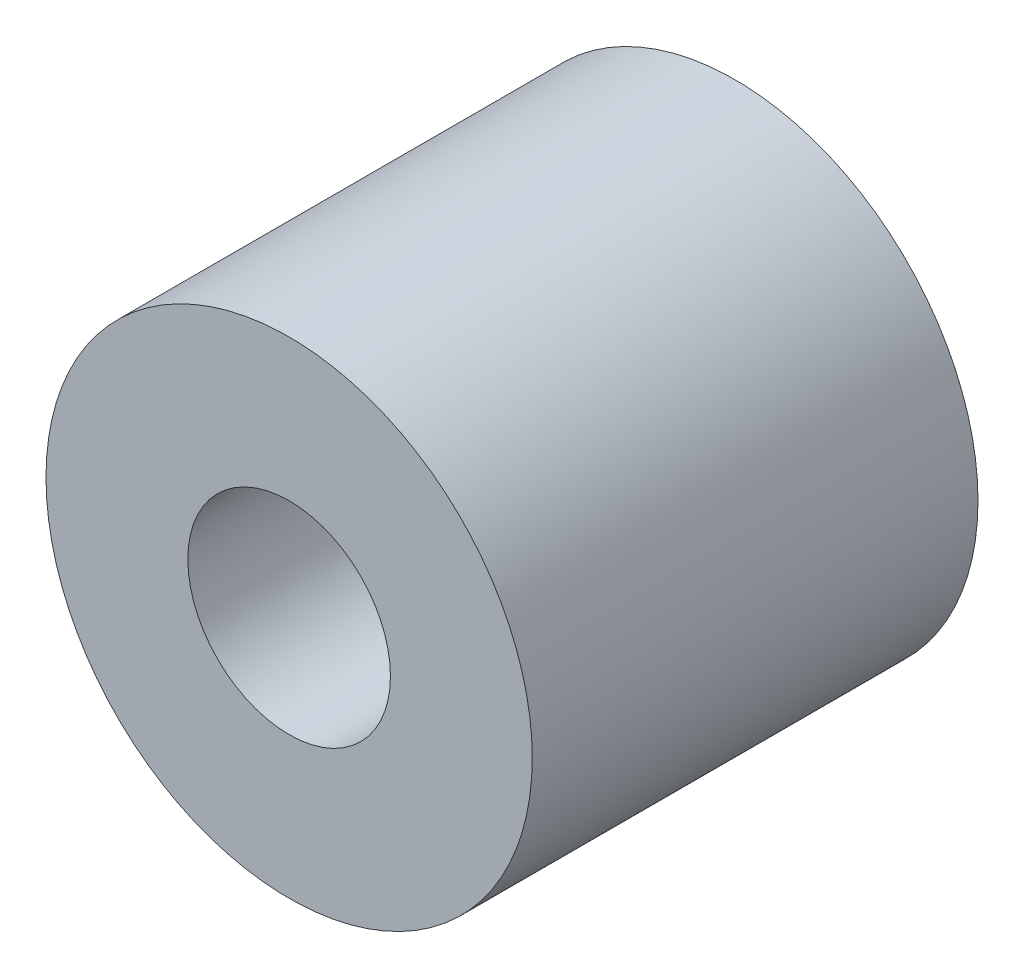
from build123d import *

# Parameters (mm, degrees)
SKETCH_1_R      = 3
SKETCH_1_R_2    = 1.25
EXTRUDE_1_DEPTH = 2.75


with BuildPart() as part:
    # 草图1 → 凸台-拉伸1 (new, symmetric)
    with BuildSketch(Plane.XY):
        Circle(SKETCH_1_R)
        Circle(SKETCH_1_R_2, mode=Mode.SUBTRACT)
    extrude(amount=EXTRUDE_1_DEPTH, both=True)


solid = part.part
